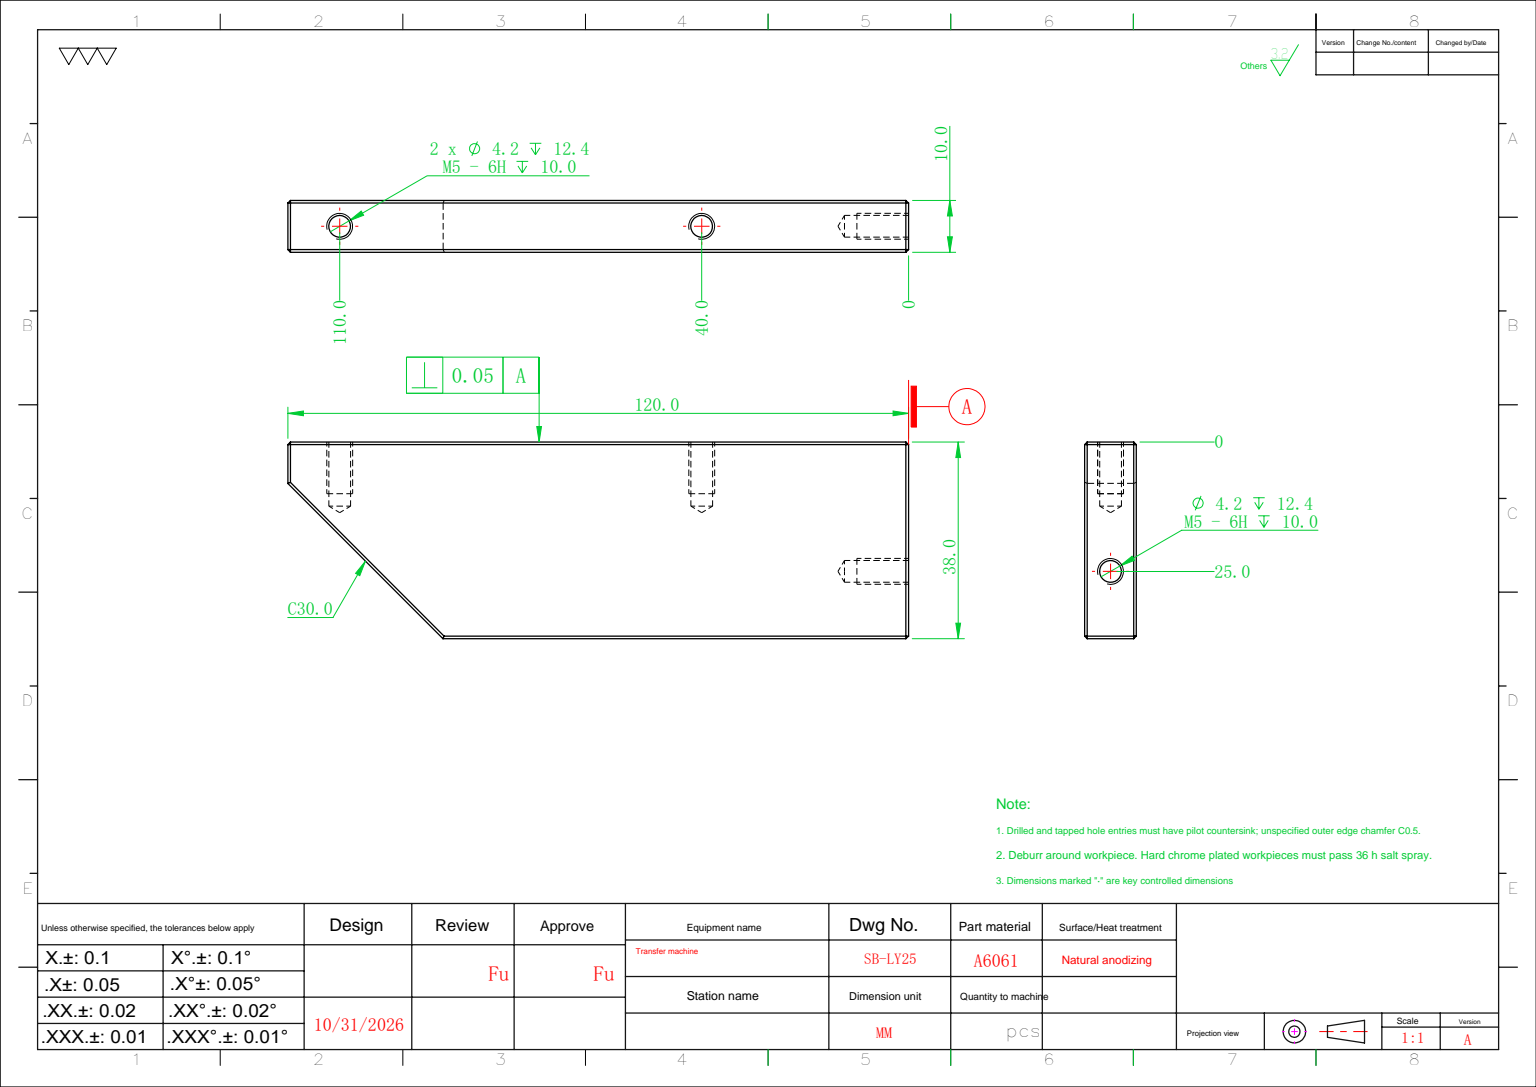
from build123d import *

# Parameters (mm, degrees)
SKETCH_1_W             = 120
SKETCH_1_H             = 38
EXTRUDE_1_DEPTH        = 10
CHAMFER_1_SIZE         = 30
HOLE_WIZARD_M5_1_D     = 4.2
HOLE_WIZARD_M5_1_DEPTH = 12.4
HOLE_WIZARD_M5_1_TIP   = 1.2618073
HOLE_WIZARD_M5_2_D     = 4.2
HOLE_WIZARD_M5_2_DEPTH = 12.4
HOLE_WIZARD_M5_2_TIP   = 1.2618073
CHAMFER_2_SIZE         = 0.5


with BuildPart() as part:
    # 草图1 → 凸台-拉伸1 (new body)
    with BuildSketch(Plane.XY):
        Rectangle(SKETCH_1_W, SKETCH_1_H)
    extrude(amount=EXTRUDE_1_DEPTH)

    # 倒角1
    chamfer_1_edges = [part.edges().sort_by_distance(p)[0] for p in [
        (60, 19, 5),
    ]]
    chamfer(chamfer_1_edges, length=CHAMFER_1_SIZE)

    # M5 螺纹孔1
    with Locations(Plane.ZY.offset(60)):
        with Locations((5, 6)):
            Hole(HOLE_WIZARD_M5_1_D / 2, depth=HOLE_WIZARD_M5_1_DEPTH)
            with Locations((0, 0, -(HOLE_WIZARD_M5_1_DEPTH + HOLE_WIZARD_M5_1_TIP / 2))):  # 118° drill point
                Cone(0, HOLE_WIZARD_M5_1_D / 2, HOLE_WIZARD_M5_1_TIP, mode=Mode.SUBTRACT)

    # M5 螺纹孔2
    with Locations(Plane(origin=(0, -19, 0), x_dir=(-1, 0, 0), z_dir=(0, -1, 0))):
        with Locations((-50, -5), (20, -5)):
            Hole(HOLE_WIZARD_M5_2_D / 2, depth=HOLE_WIZARD_M5_2_DEPTH)
            with Locations((0, 0, -(HOLE_WIZARD_M5_2_DEPTH + HOLE_WIZARD_M5_2_TIP / 2))):  # 118° drill point
                Cone(0, HOLE_WIZARD_M5_2_D / 2, HOLE_WIZARD_M5_2_TIP, mode=Mode.SUBTRACT)

    # 倒角2
    chamfer_2_edges = [part.edges().sort_by_distance(p)[0] for p in [
        (-60, 0, 10),
        (-15, 19, 0),
        (-15, 19, 10),
        (45, 4, 0),
        (45, 4, 10),
        (0, -19, 10),
        (60, -15, 10),
        (0, -19, 0),
        (-60, 0, 0),
        (60, -15, 0),
        (60, -19, 5),
        (-60, -19, 5),
        (-60, 19, 5),
    ]]
    chamfer(chamfer_2_edges, length=CHAMFER_2_SIZE)


solid = part.part
